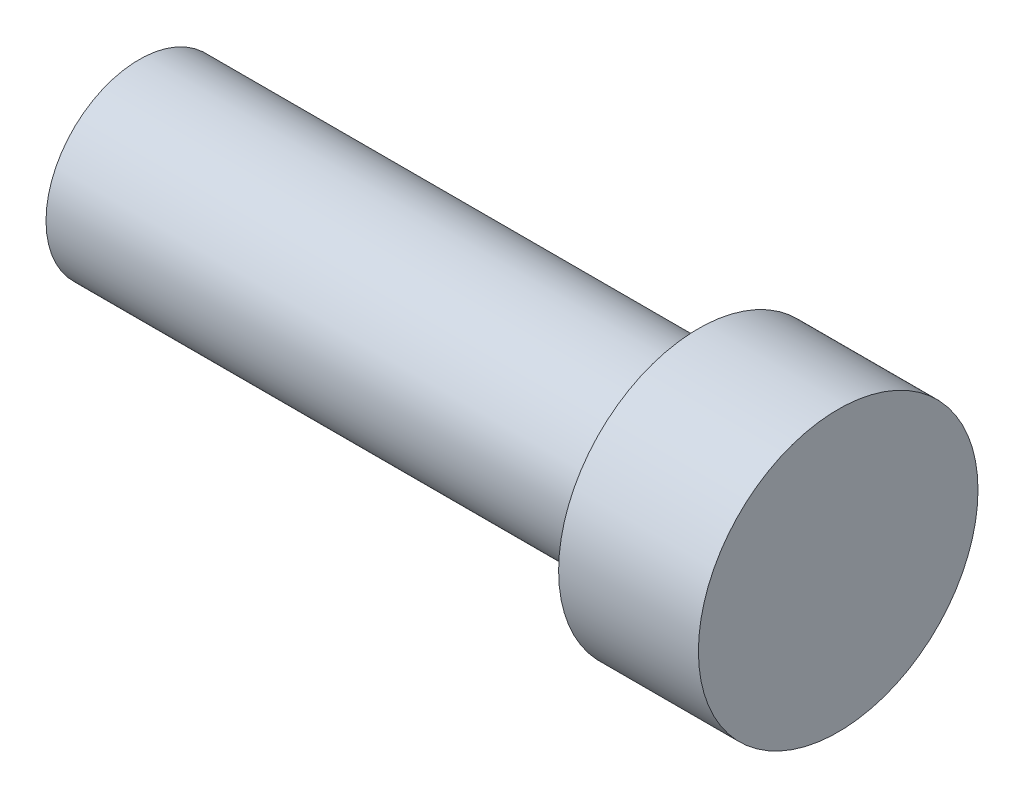
from build123d import *

# Parameters (mm, degrees)
SKETCH1_W = 12
SKETCH1_H = 2


with BuildPart() as part:
    # Sketch1 → Revolve1 (revolve)
    with BuildSketch(Plane.XY, mode=Mode.PRIVATE) as revolve1_sk:
        with Locations((1190.079016837, 96.601095303)):
            Rectangle(SKETCH1_W, SKETCH1_H)
        Polygon((1196.079016837, 98.601095303), (1196.079016837, 97.601095303), (1196.079016837, 95.601095303), (1199.079016837, 95.601095303), (1199.079016837, 98.601095303), align=None)
    revolve(revolve1_sk.sketch.rotate(Axis((1184.079016837, 95.601095303, 0), (1, 0, 0)), 90), axis=Axis((1184.079016837, 95.601095303, 0), (1, 0, 0)))


solid = part.part
